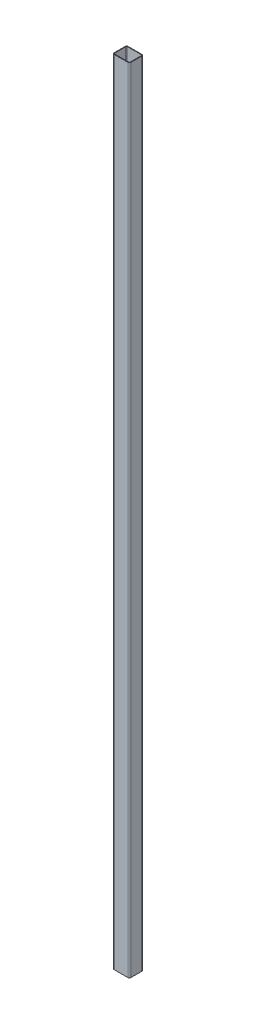
SolidWorks part; units mm, degrees
ref_plane "Front Plane" through (0, 0, 0) normal (0, 0, 1) x (1, 0, 0)
ref_plane "Top Plane" through (0, 0, 0) normal (0, 1, 0) x (1, 0, 0)
ref_plane "Right Plane" through (0, 0, 0) normal (1, 0, 0) x (0, 0, -1)
other "Configuration Table"
sketch "Sketch1" plane through (0, 0, 0) normal (0, 1, 0) x (1, 0, 0)
  line L1 (-50, 50) -> (50, 50)
  line L2 (-60, 40) -> (-60, -40)
  line L3 (-50, -50) -> (50, -50)
  line L4 (60, 40) -> (60, -40)
  line L5 (-60, 50) -> (60, -50) construction
  line L6 (-60, -50) -> (60, 50) construction
  arc A0 (50, 50) -> (60, 40) centre (50, 40) cw
  arc A1 (50, -50) -> (60, -40) centre (50, -40) ccw
  arc A2 (-60, -40) -> (-50, -50) centre (-50, -40) ccw
  arc A3 (-50, 50) -> (-60, 40) centre (-50, 40) ccw
  point P0 (0, 0)
  dimension "D3" = 10
  dimension "D1" = 120
  dimension "D2" = 100
extrude "Extrude-Thin1" add sketch "Sketch1" along normal mid plane 5702 thin
